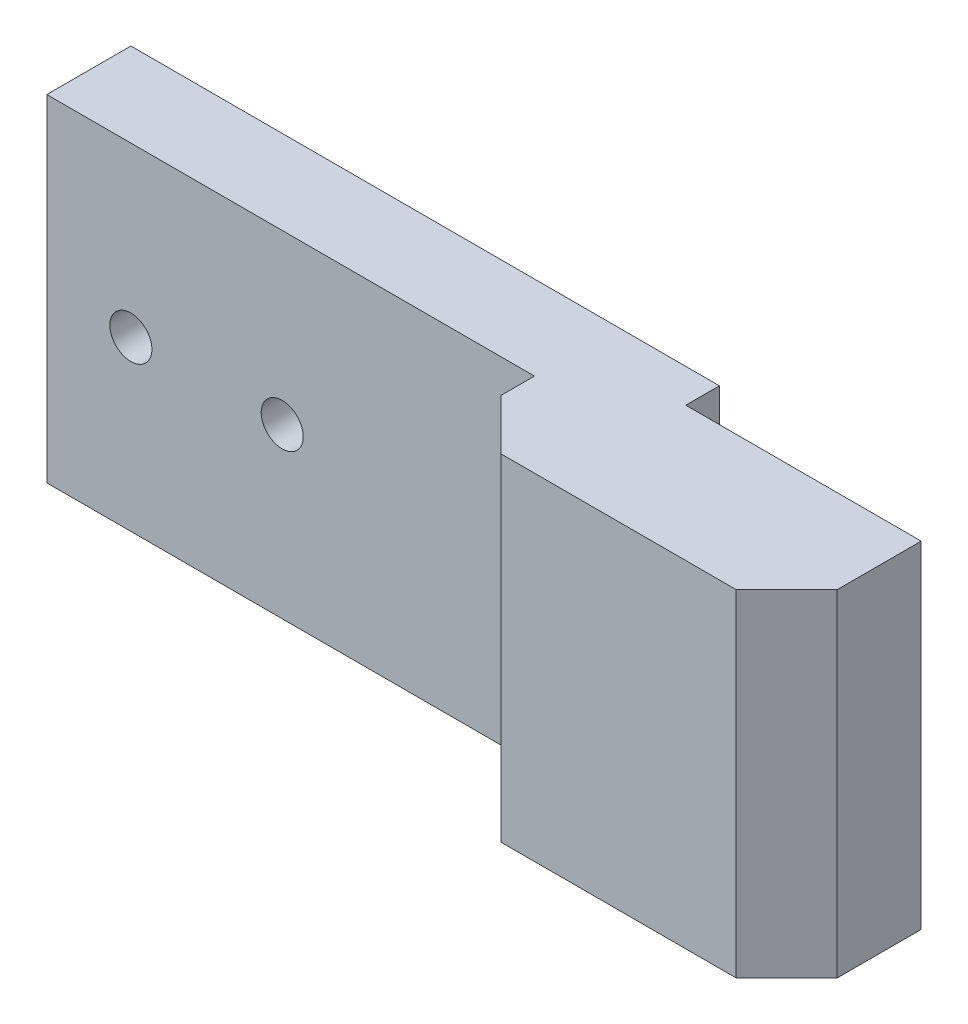
from build123d import *

# Parameters (mm, degrees)
SKETCH_1_W          = 30
SKETCH_1_H          = 20
EXTRUDE_1_DEPTH     = 5
SKETCH_2_W          = 5
SKETCH_2_H          = 20
EXTRUDE_2_DEPTH     = 5
SKETCH_4_W          = 35
SKETCH_4_H          = 10
CUT_EXTRUDE_1_DEPTH = 1
SKETCH_5_W          = 20
SKETCH_5_H          = 20
EXTRUDE_4_DEPTH     = 5
CHAMFER_1_SIZE      = 3
CHAMFER_2_SIZE      = 3
M3X0_5_1_D          = 2.5
MOVE_FACE_1_BY      = 3


with BuildPart() as part:
    # 草图1 → 凸台-拉伸1 (new body)
    with BuildSketch(Plane.XY):
        Rectangle(SKETCH_1_W, SKETCH_1_H)
    extrude(amount=EXTRUDE_1_DEPTH)

    # 草图2 → 凸台-拉伸2 (add)
    with BuildSketch(Plane(origin=(15, 0, 0), x_dir=(0, 0, -1), z_dir=(1, 0, 0))):
        with Locations((-2.5, 0)):
            Rectangle(SKETCH_2_W, SKETCH_2_H)
    extrude(amount=EXTRUDE_2_DEPTH)

    # 草图4 → 切除-拉伸1 (cut)
    with BuildSketch(Plane(origin=(0, 0, 0), x_dir=(-1, 0, 0), z_dir=(0, 0, -1))):
        with Locations((-2.5, 0)):
            Rectangle(SKETCH_4_W, SKETCH_4_H)
    extrude(amount=-CUT_EXTRUDE_1_DEPTH, mode=Mode.SUBTRACT)

    # 草图5 → 凸台-拉伸4 (add)
    with BuildSketch(Plane.XY.offset(5)):
        with Locations((24, 0)):
            Rectangle(SKETCH_5_W, SKETCH_5_H)
    extrude(amount=EXTRUDE_4_DEPTH)

    # 倒角1
    chamfer_1_edges = [part.edges().sort_by_distance(p)[0] for p in [
        (14, 0, 10),
    ]]
    chamfer(chamfer_1_edges, length=CHAMFER_1_SIZE)

    # 倒角2
    chamfer_2_edges = [part.edges().sort_by_distance(p)[0] for p in [
        (34, 0, 10),
    ]]
    chamfer(chamfer_2_edges, length=CHAMFER_2_SIZE)

    # M3x0.5 螺纹孔1 (through all)
    with Locations(Plane.XY.offset(5)):
        with Locations((-10, 0), (-1, 0)):
            Hole(M3X0_5_1_D / 2)

    # Move Face 1: a face moved outward by 3.0
    extrude(part.faces().sort_by_distance((27, 0, 5))[0], amount=MOVE_FACE_1_BY, dir=(0, 0, -1))


solid = part.part
